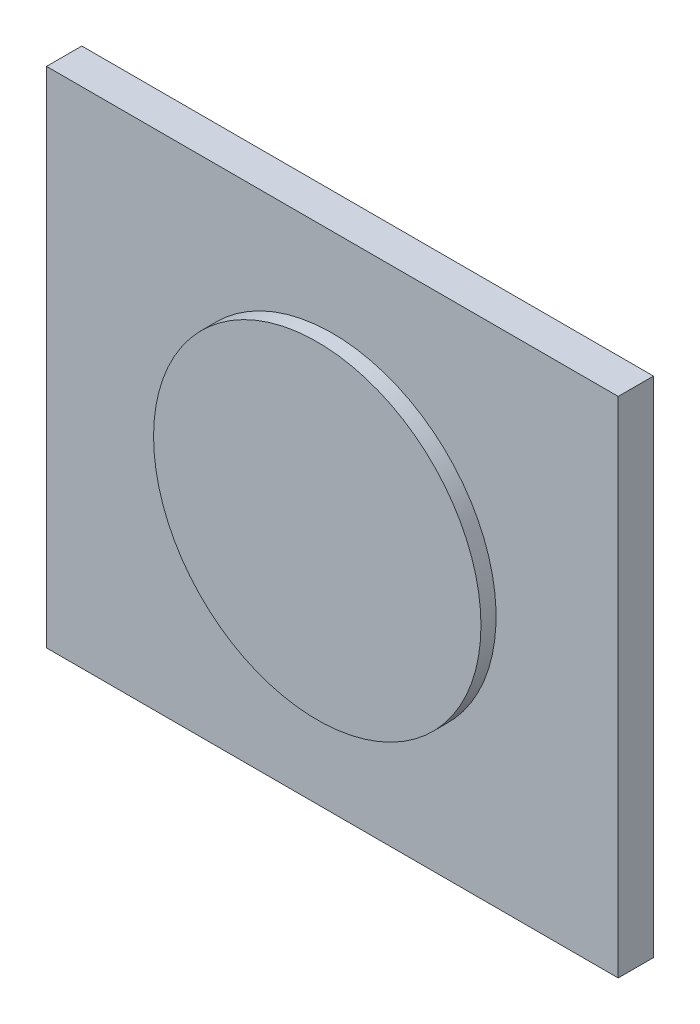
from build123d import *

# Parameters (mm, degrees)
SKETCH1_W           = 227
SKETCH1_H           = 200
BOSS_EXTRUDE1_DEPTH = 14
SKETCH2_R           = 65
BOSS_EXTRUDE2_DEPTH = 6
SKETCH3_R           = 70
BOSS_EXTRUDE3_DEPTH = 8


with BuildPart() as part:
    # Sketch1 → Boss-Extrude1 (new body)
    with BuildSketch(Plane.XY):
        with Locations((113.5, 100)):
            Rectangle(SKETCH1_W, SKETCH1_H)
    extrude(amount=BOSS_EXTRUDE1_DEPTH)

    # Sketch2 → Boss-Extrude2 (add)
    with BuildSketch(Plane.XY.offset(14)):
        with Locations(Location((113.5, 100, 0), (0, 0, 180))):
            Circle(SKETCH2_R)
    extrude(amount=BOSS_EXTRUDE2_DEPTH)

    # Sketch3 → Boss-Extrude3 (add)
    with BuildSketch(Plane(origin=(0, 0, 0), x_dir=(-1, 0, 0), z_dir=(0, 0, -1))):
        with Locations((-113.5, 100)):
            Circle(SKETCH3_R)
    extrude(amount=BOSS_EXTRUDE3_DEPTH)


solid = part.part
